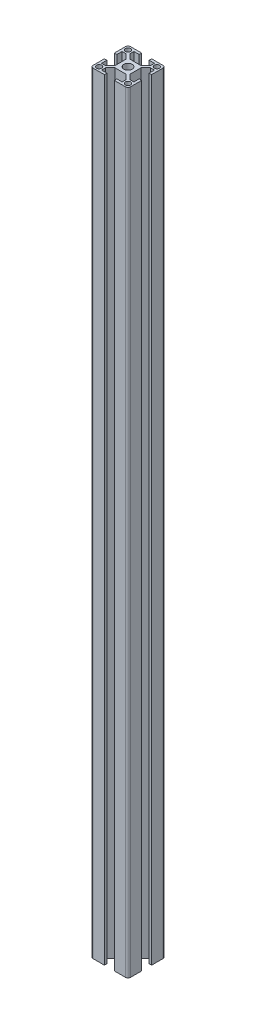
from build123d import *

# Parameters (mm, degrees)
SKETCH_1_R      = 2.1
SKETCH_1_R_2    = 3.4
EXTRUDE_1_DEPTH = 620


with BuildPart() as part:
    # 草图1 → 拉伸1 (new body)
    with BuildSketch(Plane(origin=(0, 0, 0), x_dir=(1, 0, 0), z_dir=(0, 1, 0))):
        with BuildLine():
            Line((6.75, -28), (11, -28))
            Line((11, -28), (11, -30))
            Line((11, -30), (2, -30))
            ThreePointArc((2, -30), (0.585786438, -29.414213562), (0, -28))
            Line((0, -28), (0, -19))
            Line((0, -19), (2, -19))
            Line((2, -19), (2, -23.25))
            Line((2, -23.25), (5.335785999, -23.25))
            Line((5.335785999, -23.25), (9, -19.585785999))
            Line((9, -19.585785999), (9, -10.414214001))
            Line((9, -10.414214001), (5.335785999, -6.75))
            Line((5.335785999, -6.75), (2, -6.75))
            Line((2, -6.75), (2, -11))
            Line((2, -11), (0, -11))
            Line((0, -11), (0, -2))
            ThreePointArc((0, -2), (0.585786438, -0.585786438), (2, 0))
            Line((2, 0), (11, 0))
            Line((11, 0), (11, -2))
            Line((11, -2), (6.75, -2))
            Line((6.75, -2), (6.75, -5.335785999))
            Line((6.75, -5.335785999), (10.414214001, -9))
            Line((10.414214001, -9), (19.585785999, -9))
            Line((19.585785999, -9), (23.25, -5.335785999))
            Line((23.25, -5.335785999), (23.25, -2))
            Line((23.25, -2), (19, -2))
            Line((19, -2), (19, 0))
            Line((19, 0), (28, 0))
            ThreePointArc((28, 0), (29.414213562, -0.585786438), (30, -2))
            Line((30, -2), (30, -11))
            Line((30, -11), (28, -11))
            Line((28, -11), (28, -6.75))
            Line((28, -6.75), (24.664214001, -6.75))
            Line((24.664214001, -6.75), (21, -10.414214001))
            Line((21, -10.414214001), (21, -19.585785999))
            Line((21, -19.585785999), (24.664214001, -23.25))
            Line((24.664214001, -23.25), (28, -23.25))
            Line((28, -23.25), (28, -19))
            Line((28, -19), (30, -19))
            Line((30, -19), (30, -28))
            ThreePointArc((30, -28), (29.414213562, -29.414213562), (28, -30))
            Line((28, -30), (19, -30))
            Line((19, -30), (19, -28))
            Line((19, -28), (23.25, -28))
            Line((23.25, -28), (23.25, -24.664214001))
            Line((23.25, -24.664214001), (19.585785999, -21))
            Line((19.585785999, -21), (10.414214001, -21))
            Line((10.414214001, -21), (6.75, -24.664214001))
            Line((6.75, -24.664214001), (6.75, -28))
        make_face()
        with Locations(Location((3.375, -26.625, 0), (0, 0, 270))):
            Circle(SKETCH_1_R, mode=Mode.SUBTRACT)
        with Locations(Location((26.625, -26.625, 0), (0, 0, 270))):
            Circle(SKETCH_1_R, mode=Mode.SUBTRACT)
        with Locations(Location((15, -15, 0), (0, 0, 270))):
            Circle(SKETCH_1_R_2, mode=Mode.SUBTRACT)
        with Locations(Location((3.375, -3.375, 0), (0, 0, 270))):
            Circle(SKETCH_1_R, mode=Mode.SUBTRACT)
        with Locations(Location((26.625, -3.375, 0), (0, 0, 270))):
            Circle(SKETCH_1_R, mode=Mode.SUBTRACT)
    extrude(amount=EXTRUDE_1_DEPTH)


solid = part.part
